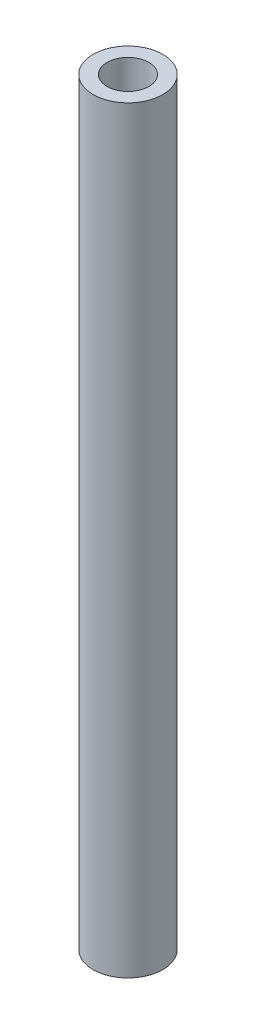
from build123d import *

# Parameters (mm, degrees)
SKETCH1_R           = 2.5
SKETCH1_R_2         = 1.5
BOSS_EXTRUDE1_DEPTH = 54.4
SKETCH2_R           = 1.5
SKETCH2_R_2         = 0.5
BOSS_EXTRUDE2_DEPTH = 2


with BuildPart() as part:
    # Sketch1 → Boss-Extrude1 (new body)
    with BuildSketch(Plane(origin=(0, 0, 0), x_dir=(1, 0, 0), z_dir=(0, 1, 0))):
        with Locations(Location((0, 0, 0), (0, 0, 270))):
            Circle(SKETCH1_R)
        with Locations(Location((0, 0, 0), (0, 0, 270))):
            Circle(SKETCH1_R_2, mode=Mode.SUBTRACT)
    extrude(amount=BOSS_EXTRUDE1_DEPTH)

    # Sketch2 → Boss-Extrude2 (add)
    with BuildSketch(Plane.XZ):
        with Locations(Location((0, 0, 0), (0, 0, 270))):
            Circle(SKETCH2_R)
        with Locations(Location((0, 0, 0), (0, 0, 270))):
            Circle(SKETCH2_R_2, mode=Mode.SUBTRACT)
    extrude(amount=-BOSS_EXTRUDE2_DEPTH)


solid = part.part
